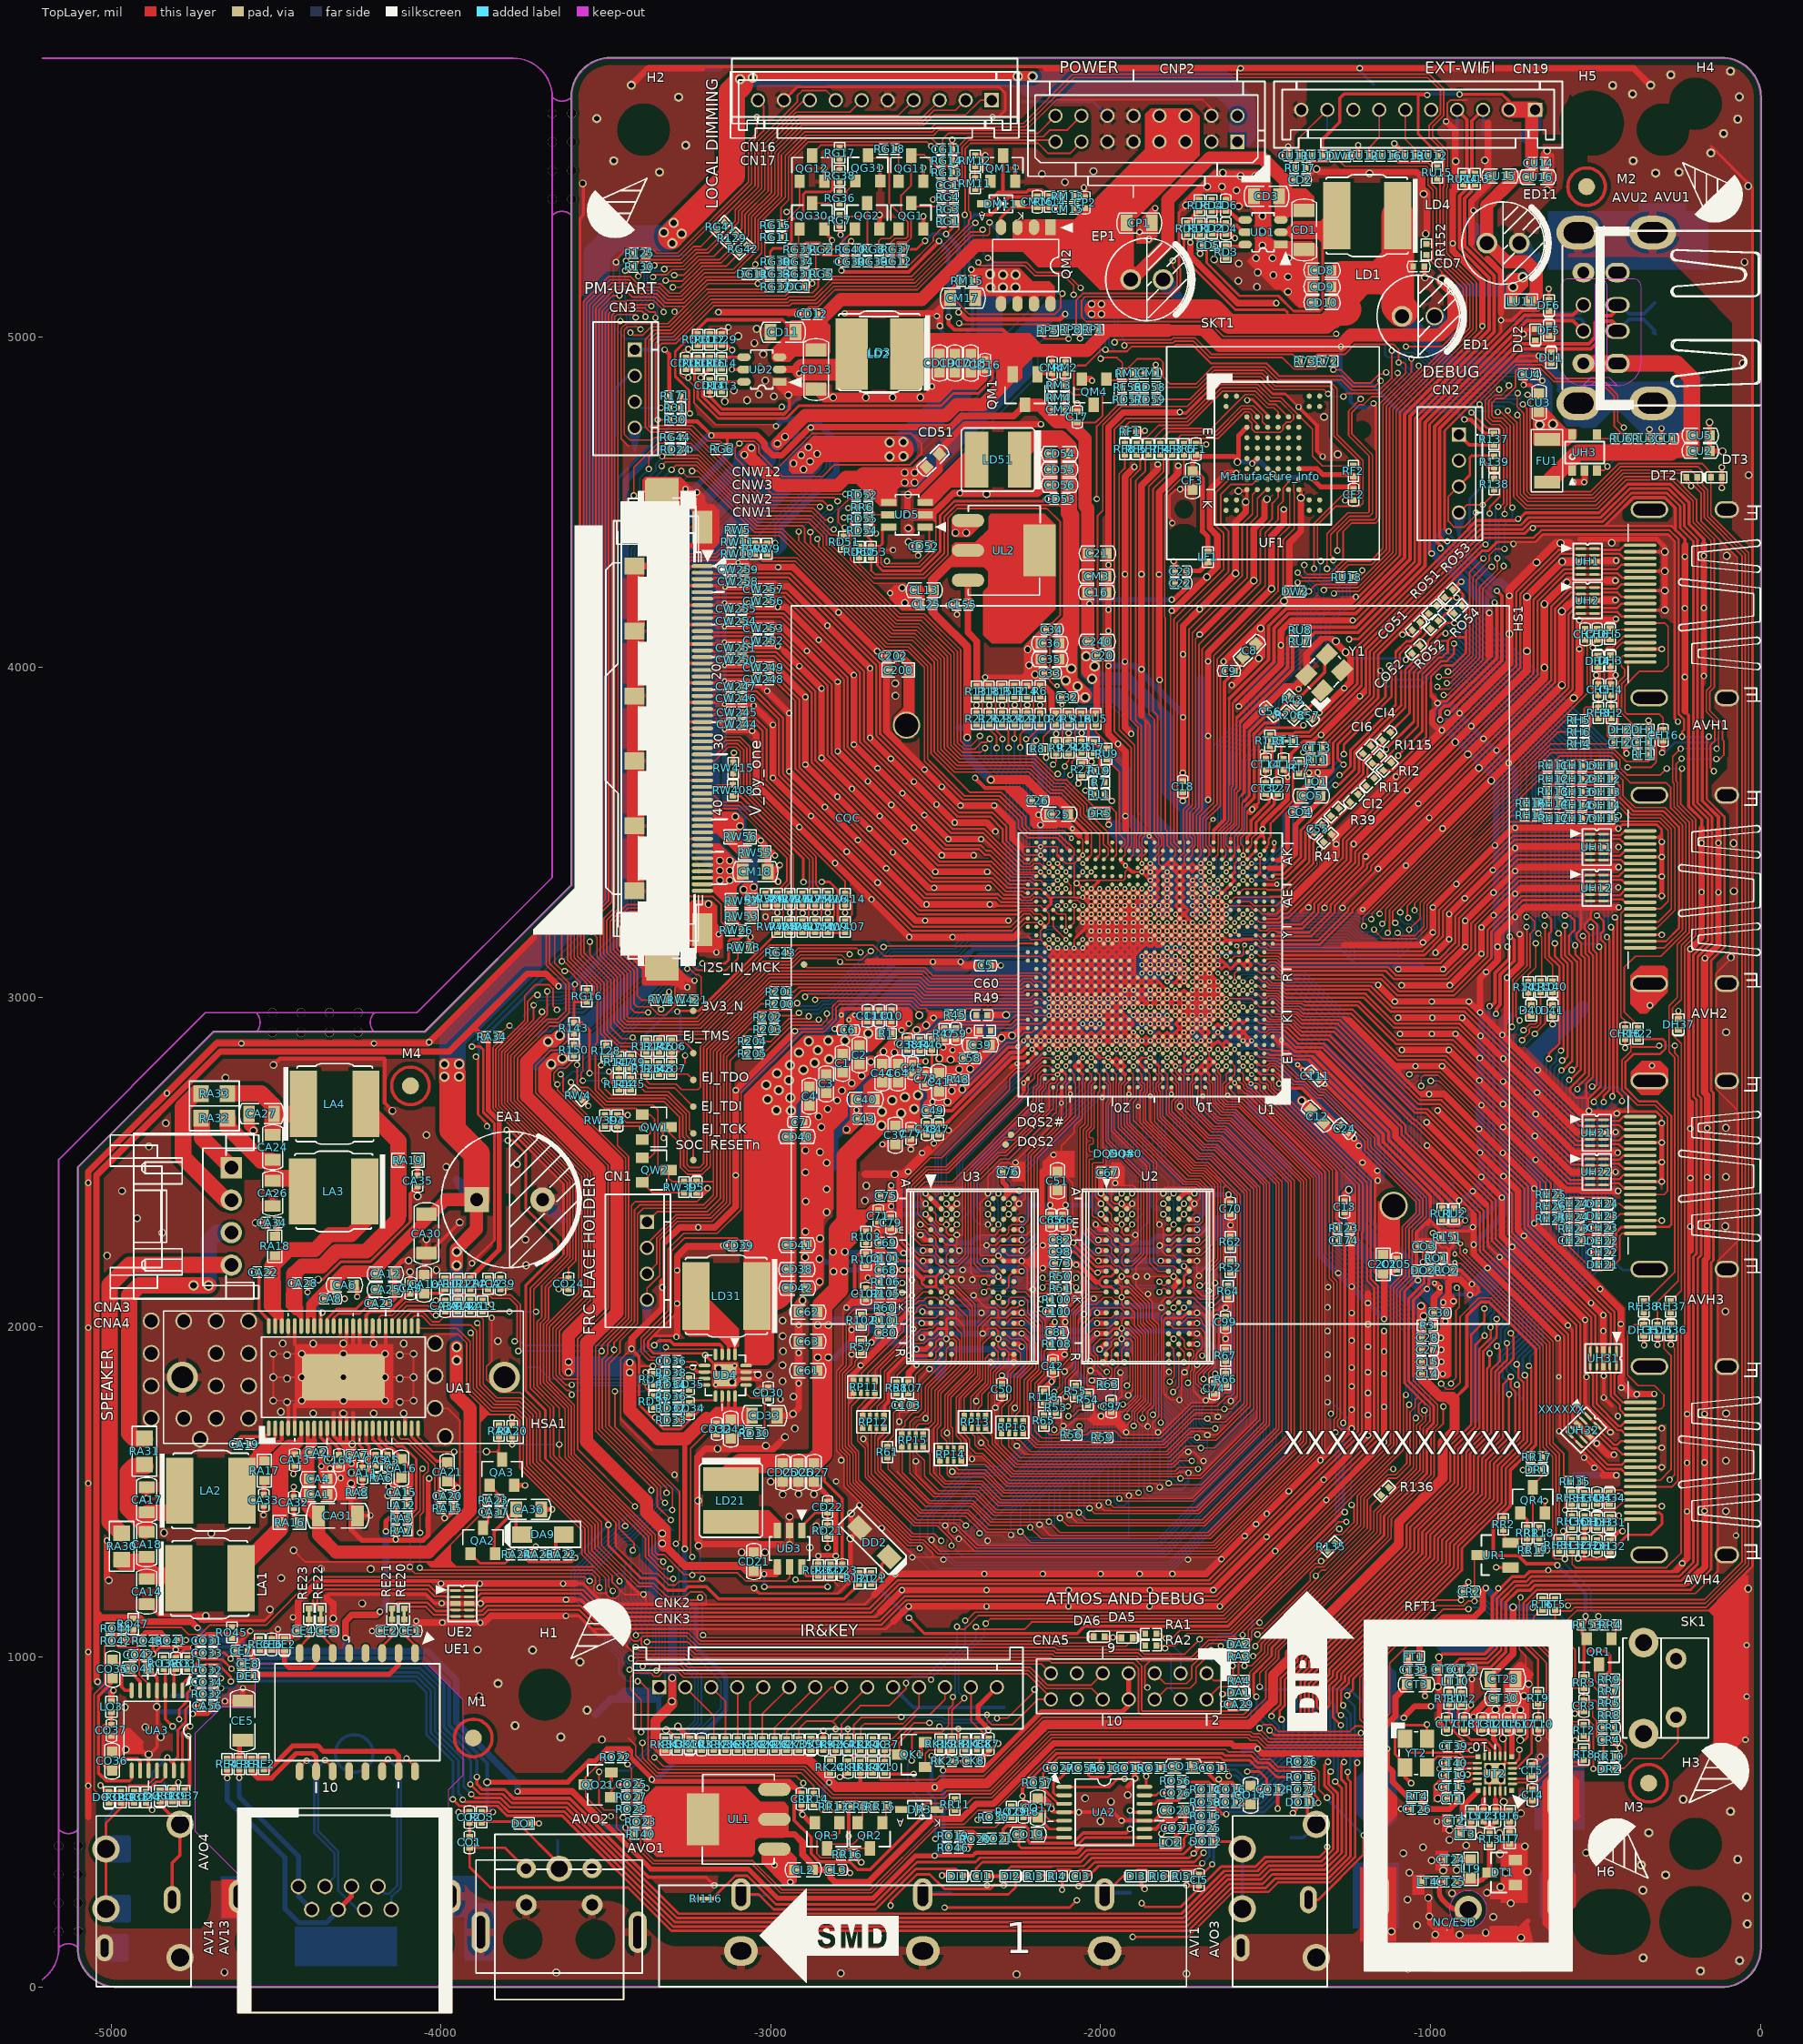
[diagram p0: TopLayer view]
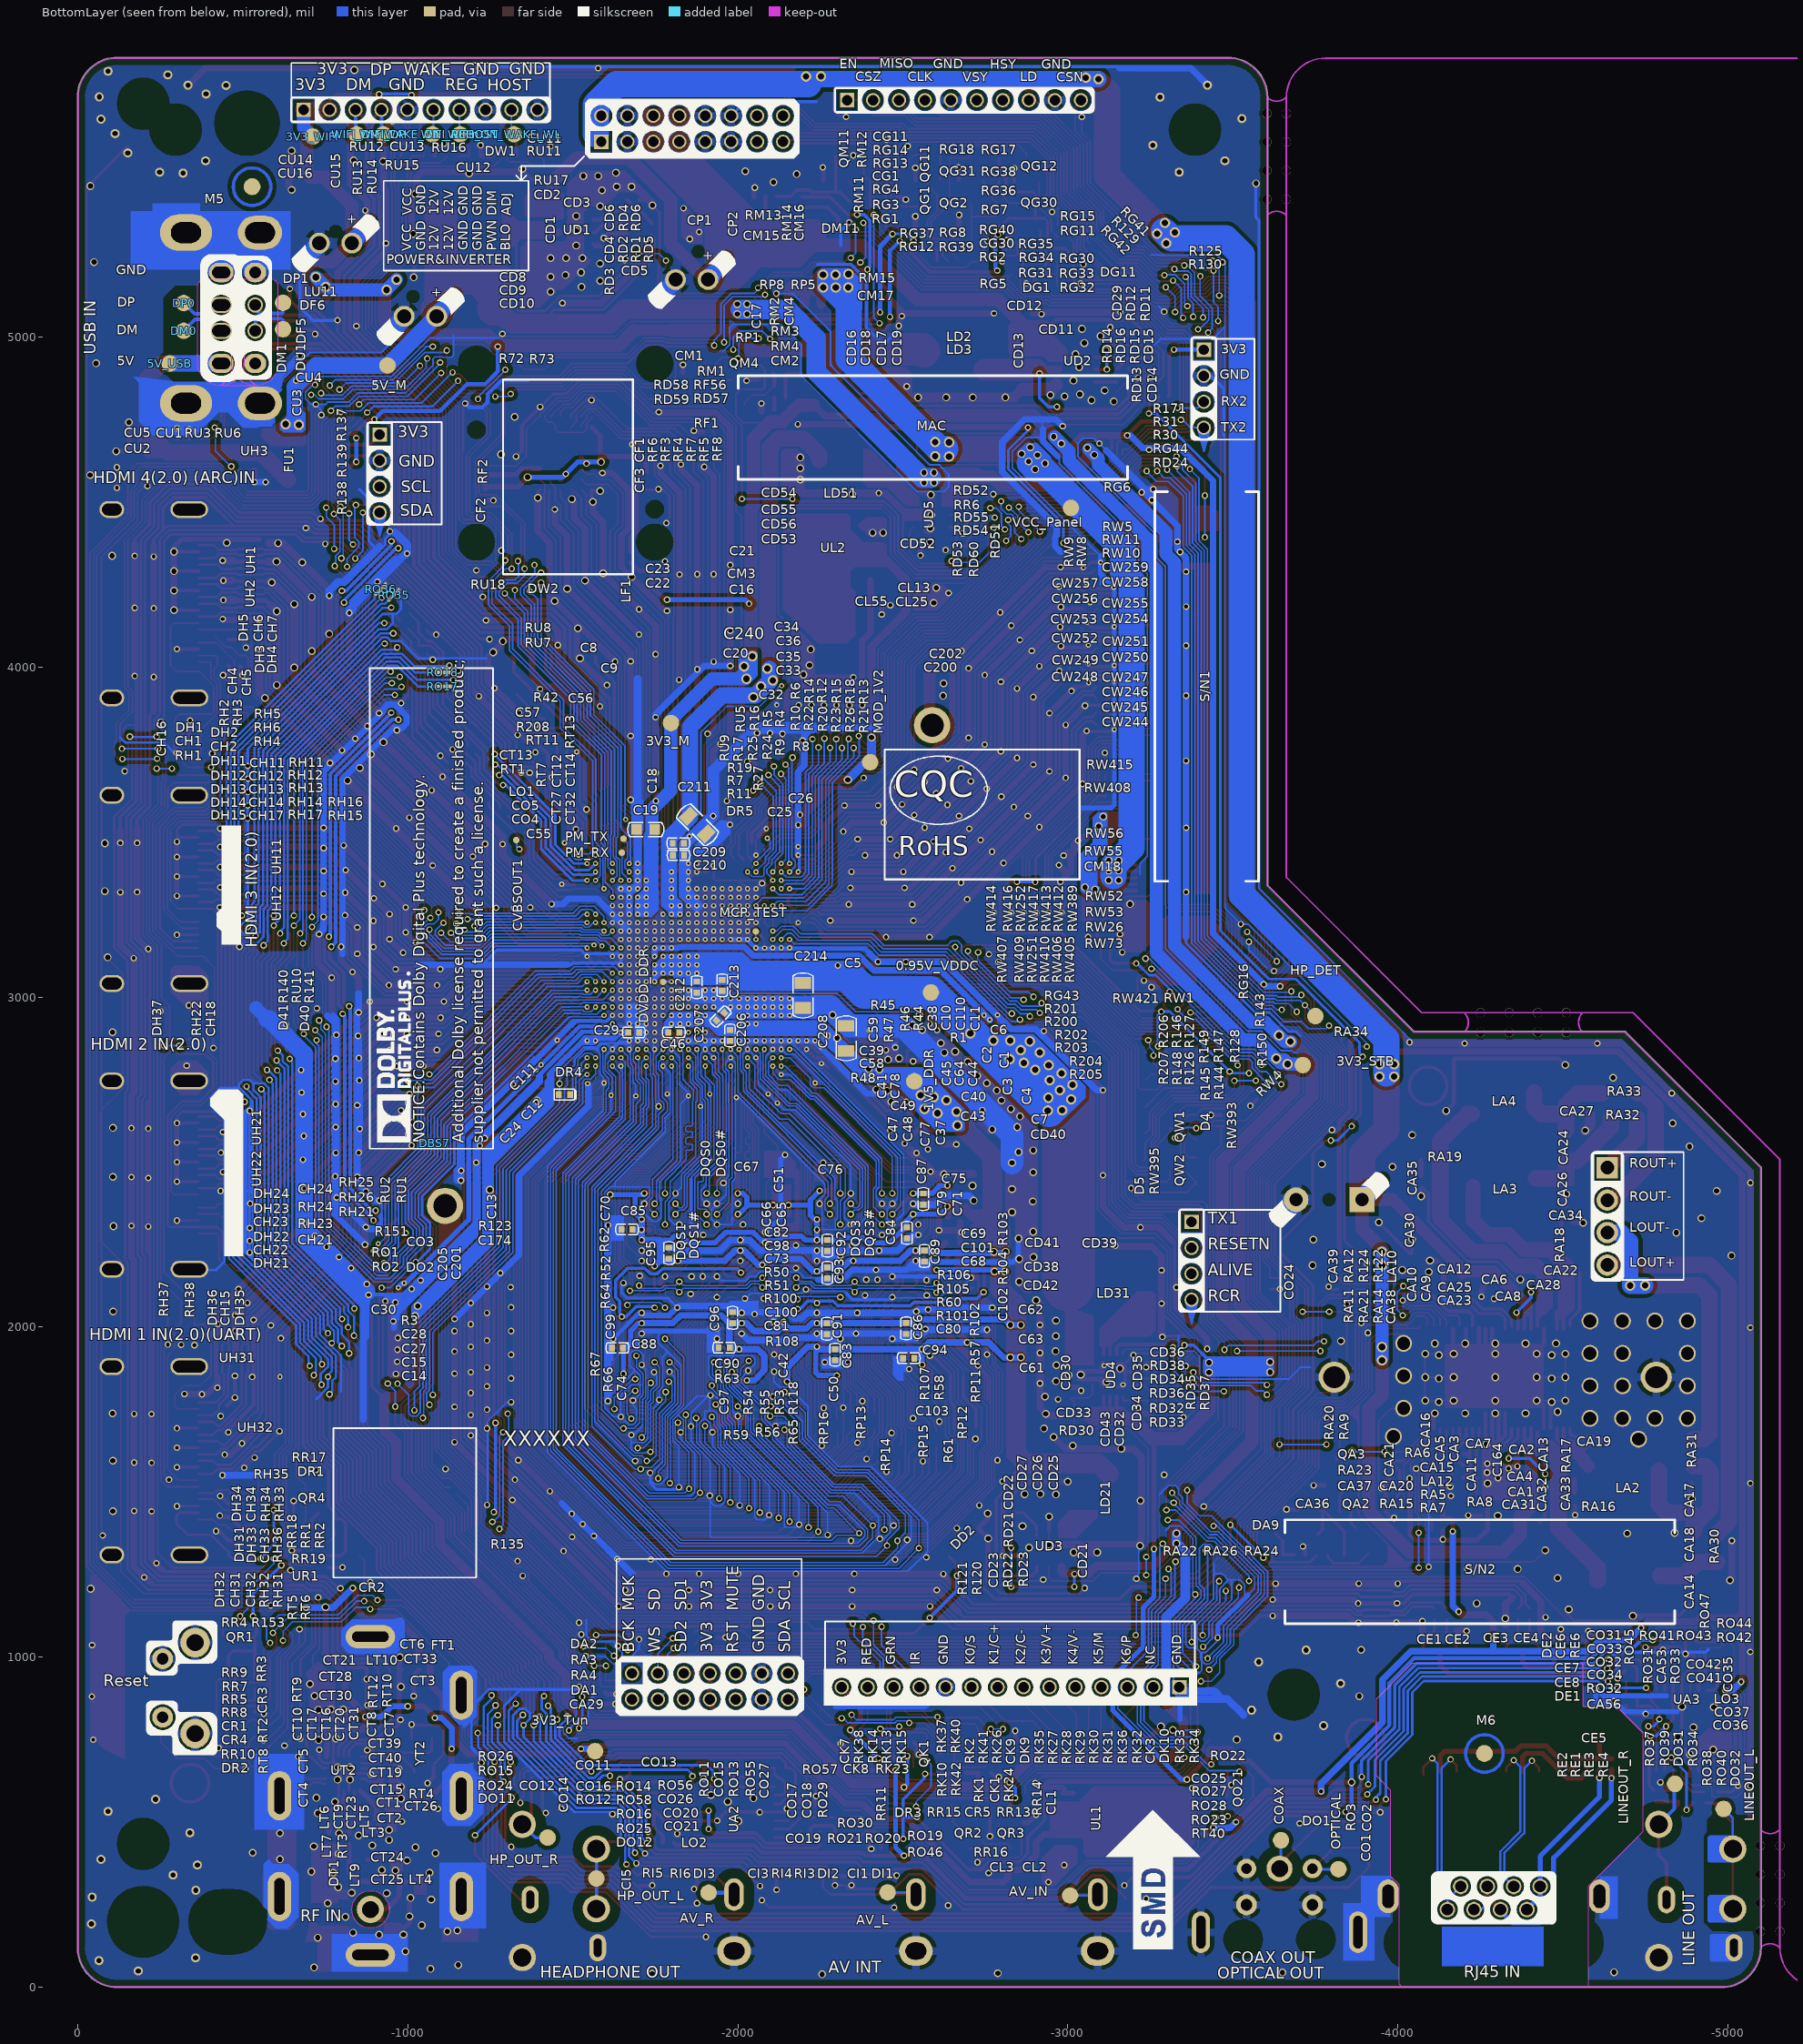
[diagram p1: BottomLayer view, seen from below]
# Altium PCB MISC86290.PcbDoc (part 1 of 31)
Units mil, origin at the board's own origin, x right, y up, seen from the top; angles counter-clockwise.
Board outline 5104.71 x 5851.49 mil, 2 copper layers (TopLayer, BottomLayer), stack 61.855 mil thick; 1026 components, 667 nets, 4280 pads, 2294 vias.

## Layer stack, top to bottom
TopLayer: signal copper 1.4
Dielectric: core 59.055, FR-4, Dk 4.8
BottomLayer: signal copper 1.4

## Board outline
-5102.19,118.11 ccw(c-4981.57,118.11) -4981.57,-2.52 ccw(c-4981.57,0) -4980.94,-2.44 ccw(c-4980.32,0) -4980.32,-2.51 -118.11,-2.51 ccw(c-118.11,0) -118.07,-2.51 ccw(c-118.11,118.11) 2.51,118.07 ccw(c-118.11,118.11) 2.51,118.11 2.51,5728.35 ccw(c-118.11,5728.35) -118.11,5848.97 ccw(c-118.11,5846.46) -118.2,5848.97 -3484.25,5848.97 ccw(c-3484.25,5846.46) -3484.88,5848.89 ccw(c-3485.5,5846.46) -3485.5,5848.97 ccw(c-3485.5,5728.35) -3606.13,5728.35 -3606.13,3339.68 -4049.59,2896.21 -4689.25,2896.21 ccw(c-4689.25,2893.7) -4689.29,2896.21 ccw(c-4689.33,2893.7) -4691.11,2895.48 -5101.45,2485.13 ccw(c-5099.67,2483.36) -5102.19,2483.36 -5102.19,118.23 ccw(c-5099.68,118.11)

## Design rules (kind name [scope] priority, off if disabled: settings)
Clearance ■KEEPOUT_18mil [(IsTrack Or IsArc) And (AsMM(Width) < 1) And IsKeepOut vs Not IsPad] p1: gap=18
Clearance ■DFM_NPTH_10mil [(IsPadHoleValid And (PadIsPlated=false) Or IsPad And ((AsMM(PadXSize_AllLayers) < 1) or (AsMM(PadYSize_AllLayers) < 1 )) And IsKeepout) OR HasFootprintPad('ASSE*','0') vs Not IsPad] p2: gap=10
Clearance ■DFM_20mil [(IsTrack or IsArc or IsPad) And IsKeepOut vs IsTrack or IsArc or InPoly] p3: gap=20
Clearance ■PWR_A12_8mil [(InNetClass('PWR_A12_8mil') or InNet('*12V*') or InNet('*24V*') or InNet('*PVCC*') or InNet('*19V*') or InNet('*AMP*POWER*') or InNet('*AMP*VCC*') or InNet('*LNB*')) and Not IsPad vs Not InPoly] p4: gap=8
Clearance ■SIP2GND_8mil [HasFootprint('SIP*') vs InPoly] p5: gap=8
Clearance ■Poly_4mil [InPolygonClass('Poly_4mil') vs Not InPoly] p6: gap=4
Clearance ■Poly_5mil [InPolygonClass('Poly_5mil') vs Not InPoly] p7: gap=5
Clearance ■Poly_8mil [InPolygonClass('Poly_8mil') vs Not InPoly] p8: gap=8
Clearance ■ESD_10mil [HasFootprint('*IEC*') Or HasFootprint('*-F1*') Or HasFootprint('ANT-RF*')] p9: gap=10
Clearance ■ESD_20mil [HasFootprint('*SHIELD*')] p10: gap=20
Clearance ■C_RFGND_1.8mm [InNet('RFGND') vs Not (InNet('RF*IN*') OR InNet('NetCT28*'))] p11: gap=70.87
Clearance ■GND_12mil [InNet('GND') vs InPoly] p12: gap=12
Clearance ■ESD_30mil [(HasFootprint('SCART*') OR HasFootprint('AV*') OR HasFootprint('DB15*') OR HasFootprint('PHONE*')) vs OnBottomLayer] p13: gap=30
Clearance ■ESD_NT_30mil [HasFootprint('SCART*') Or HasFootprint('PHONE-HD-12') Or HasFootprint('PHONE-HD-17') Or HasFootprint('PHONE-HD-10') Or HasFootprint('PHONE-HD-26') vs InNet('GND') And OnTopLayer] p14: gap=30
Clearance ■DFM_TH_5mil [HasFootprint('GND') or HasFootprint('TP*') or HasFootprint('MARK*') or HasFootprint('SPARK_GAP') or HasFootprint('USB-HD-3-2') or HasFootprint('PHONE-HS-20') and Not IsRegion vs OnBottomlayer And IsPad OR IsPadHoleValid] p15: gap=5
Clearance ■DFM_HS60_5mil [InPadClass('HS60') vs InPadClass('HS60') OR IsPadHoleValid and not InPadClass('VIA5')] p16: gap=5
Clearance ■DFM_BCR_4mm [IsPadHoleValid vs IsBoardCutoutRegion] p17: gap=157.48
Clearance ■DFM_TH_4mm [OnBottomlayer And IsSMTPin vs IsPadHoleValid and not InPadClass('VIA5')] p18: gap=157.48
Clearance ■DFM_HS60_4mm [InPadClass('HS60') vs IsPad and OnBottomlayer] p19: gap=157.48
Clearance ■VIA2VIA_6.2mil [(IsVia OR InPadClass('VIA5')) And Not (IsVia And (AsMM(HoleDiameter) = 0.1)) vs (IsVia OR InPadClass('VIA5')) And Not (IsVia And (AsMM(HoleDiameter) = 0.1))] p20: gap=6.2
Clearance ■VIA2VIA_9.8mil [(IsVia OR InPadClass('VIA5')) And Not (IsVia And (AsMM(HoleDiameter) = 0.1)) vs (IsVia OR InPadClass('VIA5')) And Not (IsVia And (AsMM(HoleDiameter) = 0.1))] p21: gap=9.8
Clearance ■VIA2PAD_BGA_3.9mil [HasFootprint('BGA*') and IsPad vs (IsVia OR InPadClass('VIA5')) And Not (IsVia And (AsMM(HoleDiameter) = 0.1))] p22: gap=3.9
Clearance ■VIA2PAD_5mil [IsVia And Not (IsVia And (AsMM(HoleDiameter) = 0.1)) vs ISPAD and Not HasFootprintPad('*','EPAD') and Not HasFootprintPad('*','257') and Not HasFootprintPad('TP','*') and Not HasFootprintPad('GND','JP*') and Not HasFootprintPad('LQFP216/0.4-2','217') and Not HasFootprintPad('QFP16*','17') and Not HasFootprintPad('QFN16*','17') and Not HasFootprintPad('QFN20*','21') and Not HasFootprintPad('QFN24*','25') and Not HasFootprintPad( 'QFN24*','29') and Not HasFootprintPad('QFN28*','29') and Not HasFootprintPad('QFN32*','33') and Not HasFootprintPad('QFN36*','37') and Not HasFootprintPad('QFN36*','0') and Not HasFootprintPad('QFN32*','0') and Not HasFootprintPad('QFN40*','41') and Not HasFootprintPad('QFN48*','49') and Not HasFootprintPad('LQFP48/0.5-2','49') and Not HasFootprintPad('*SSOP32*','33') and Not HasFootprintPad('SOP8*','9') and Not HasFootprintPad('WSON8/1.27*','9') and Not HasFootprintPad('DFN10/0.5-1*','11') and Not HasFootprintPad('SON16/0.4','9') and Not HasFootprintPad('MSOP10/0.5-1','11') and Not HasFootprintPad('QFN56/0.5','57') and Not HasFootprintPad('LGA31/0.5','3*') and Not InPadClass('VIA_HS60') and Not HasFootprintPad('TSSOP16/0.65-3','17') and Not HasFootprintPad('QFP128/0.5-2','129') and Not HasFootprintPad('QFP128/0.4-5','129') and Not HasFootprintPad('PQFP48*','49') and Not HasFootprintPad('QFP156/0.4-1','157')] p23: gap=5
Clearance ■PAD2VIA5_6mil [IsPad And ((AsMM(PadXSize_AllLayers) < 2.5) or ((AsMM(PadYSize_AllLayers) < 2.5))) And Not InPadclass('HS60') vs InPadClass('VIA5')] p24: gap=6
Clearance "■12mil for Polygon" [InPoly] p25: gap=12
Clearance 8mil [All] p26 off: gap=8
Clearance 7mil [All] p27 off: gap=7
Clearance 6.2mil [All] p28 off: gap=6.2
Clearance 6mil [All] p29 off: gap=6
Clearance 5.8mil [All] p30 off: gap=5.8
Clearance 5mil [Not ((IsTrack Or IsArc) And (Layer = 'KeepOutLayer')) vs Not (IsPad or ((IsTrack Or IsArc) And (Layer = 'KeepOutLayer')))] p31 off: gap=5
Clearance 4.5mil [Not ((IsTrack Or IsArc) And (Layer = 'KeepOutLayer')) vs Not (IsPad or ((IsTrack Or IsArc) And (Layer = 'KeepOutLayer')))] p32 off: gap=4.5
Clearance "3.9mil for Minimum" [Not ((IsTrack Or IsArc) And (Layer = 'KeepOutLayer')) vs Not (IsPad or ((IsTrack Or IsArc) And (Layer = 'KeepOutLayer')))] p33: gap=3.9
ComponentClearance [All] p1 off: gap=0.1 collisioncheckmode=3 verticalgap=39.37 showdistances=FALSE
DiffPairsRouting DiffPair_USB_DiffPairsRouting [InDifferentialPairClass('USB')] p1: maxlimit=5 minlimit=4 mostfreqgap=5 maxuncoupledlength=200
DiffPairsRouting DiffPair_LVDS_DiffPairsRouting [InDifferentialPairClass('LVDS')] p2: maxlimit=5 minlimit=4 mostfreqgap=5 maxuncoupledlength=500
DiffPairsRouting DiffPair_HDMI_DiffPairsRouting [InDifferentialPairClass('HDMI')] p3: maxlimit=5 minlimit=4 mostfreqgap=5 maxuncoupledlength=200
DiffPairsRouting [All] p4: maxlimit=10 minlimit=10 mostfreqgap=10 maxuncoupledlength=500
FabricationTestPointUsage TestPointUsage [All] p1: valid=0 allowmultiple=FALSE
FabricationTestpoint Testpoint [All] p1: side=3 testpointundercomponent=TRUE minsize=40 maxsize=100 preferedsize=60 minholesize=20 maxholesize=40 preferedholesize=32 testpointgrid=1 allowsidetop=TRUE allowsidebottom=TRUE usegrid=TRUE gridtolerance=0.01
HoleSize HoleSize_VIA [ISVIA] p1 off: absolutevalues=TRUE maxlimit=23.62 minlimit=7.87 maxpercent=80.000 minpercent=20.000
HoleToHoleClearance Hole2Hole [All] p1 off: gap=18 allowstackedmicrovias=FALSE
MatchedLengths DiffPair_USB_MatchedLengths [InDifferentialPairClass('USB')] p1: tolerance=100 checknetsindiffpair=TRUE checkdiffpairvsdiffpair=FALSE checkothers=FALSE
MatchedLengths DiffPair_LVDS_MatchedLengths [InDifferentialPairClass('LVDS')] p2: tolerance=100 checknetsindiffpair=TRUE checkdiffpairvsdiffpair=FALSE checkothers=FALSE
MatchedLengths DiffPair_HDMI_MatchedLengths [InDifferentialPairClass('HDMI')] p3: tolerance=100 checknetsindiffpair=TRUE checkdiffpairvsdiffpair=FALSE checkothers=FALSE
MinimumAnnularRing [All] p1: minimumring=3.94
MinimumSolderMaskSliver [All] p1 off: minsoldermaskwidth=-1
NetAntennae [Not (HasFootprint('ANT-7') or HasFootprint('ANT-BLUECORE'))] p1: netantennaetolerance=40
PermittedLayers [All] p1: toplayerpermitted=TRUE bottomlayerpermitted=TRUE
PlaneClearance Plane_ESD_30mil [(HasFootprint('SCART*') OR HasFootprint('AV*') OR HasFootprint('DB15*') OR HasFootprint('PHONE*'))] p1: clearance=30
PlaneClearance [All] p2: clearance=9
PlaneConnect Plane2Via [IsVia or InPadClass('VIA5')] p1: planeconnectstyle=Direct reliefexpansion=20 reliefentries=4 reliefconductorwidth=10 reliefairgap=10
PlaneConnect PlaneConnect_PAD [HasFootprint('ASSE*') OR InPadclass('HS60')] p2: planeconnectstyle=Direct reliefexpansion=20 reliefentries=4 reliefconductorwidth=10 reliefairgap=10
PlaneConnect [All] p3: planeconnectstyle=Relief reliefexpansion=12 reliefentries=4 reliefconductorwidth=30 reliefairgap=12
PolygonConnect PourOverVia [IsVia vs IsPolygon] p1: connectstyle=Direct reliefconductorwidth=10 reliefentries=4 polygonreliefangle="90 Angle"
PolygonConnect VIA5_HS60 [InPadclass('HS60') or InPadClass('VIA5') vs IsPolygon] p2: connectstyle=Direct reliefconductorwidth=10 reliefentries=4 polygonreliefangle="90 Angle"
PolygonConnect Polygon_RFGND [InNet('RFGND')] p3: connectstyle=Direct reliefconductorwidth=10 reliefentries=4 polygonreliefangle="90 Angle"
PolygonConnect ESD_SCART [HasFootprint('SCART*') vs IsPolygon And onBottomlayer] p4: connectstyle=Direct reliefconductorwidth=30 reliefentries=4 polygonreliefangle="90 Angle"
PolygonConnect FH2Polygon [HasFootprint('ASSE*') or HasFootprint('DIODE-S0402') or HasFootprint('RCL0524P') vs IsPolygon] p5: connectstyle=Direct reliefconductorwidth=10 reliefentries=4 polygonreliefangle="90 Angle"
PolygonConnect PWC1_2Polygon [(HasFootprint('*0805*') OR HasFootprint('*1206*')) vs IsPolygon] p6: connectstyle=Relief reliefconductorwidth=30 reliefentries=4 polygonreliefangle="90 Angle"
PolygonConnect PWC2_2Polygon [HasFootprint('*0603*') vs IsPolygon] p7: connectstyle=Relief reliefconductorwidth=25 reliefentries=4 polygonreliefangle="90 Angle"
PolygonConnect PWC3_2Polygon [HasFootprint('EC*') vs IsPolygon] p8: connectstyle=Relief reliefconductorwidth=35 reliefentries=4 polygonreliefangle="90 Angle"
PolygonConnect PWC2Polygon [(HasFootprint('SOT-89') OR HasFootprint('SOT-223') OR HasFootprint('TO-252') OR HasFootprint('TO-263') OR HasFootprint('DIODE') OR HasFootprint('SW-HS-2') OR HasFootprint('HDMI*') OR HasFootprint('SO-8B') OR HasFootprint('GND') OR HasFootprint('PHONE*') OR HasFootprint('DIP18/2.54-2') OR HasFootprint('DIP18/2.54-1') OR HasFootprint('UFL-R-SMT-1') OR HasFootprint('WIFI') OR HasFootprint('UM02BS') OR HasFootprint('*SCART*') OR HasFootprint('TSOT23-8/0.65') OR HasFootprint('*SOT-23-*') OR HasFootprint('SOP23-5-1') OR HasFootprint('SOP6/0.95') OR HasFootprint('M-WIFI-2-M603USA1') OR HasFootprint('M-MT7632U') OR HasFootprint('SOP8/1.27') OR HasFootprint('SOP8/1.27-3')) vs IsPolygon] p9: connectstyle=Direct reliefconductorwidth=35 reliefentries=4 polygonreliefangle="90 Angle"
PolygonConnect SMD2Polygon [IsSMTPin vs IsPolygon] p10: connectstyle=Relief reliefconductorwidth=12 reliefentries=4 polygonreliefangle="90 Angle"
PolygonConnect PTH2Polygon [IsThruPin vs IsPolygon] p11: connectstyle=Relief reliefconductorwidth=25 reliefentries=4 polygonreliefangle="90 Angle"
RoutingVias 0.6_0.4 [All] p1 off: holewidth=15.75 width=23.62 viastyle="Through Hole" minholewidth=15.75 minwidth=23.62 maxholewidth=15.75 maxwidth=23.62
RoutingVias 0.8_0.5 [All] p2 off: holewidth=19.68 width=31.5 viastyle="Through Hole" minholewidth=19.68 minwidth=31.5 maxholewidth=19.68 maxwidth=31.5
RoutingVias 0.5_0.3 [All] p3: holewidth=11.81 width=19.68 viastyle="Through Hole" minholewidth=11.81 minwidth=19.68 maxholewidth=11.81 maxwidth=19.68
RoutingVias 0.45_0.25 [All] p4 off: holewidth=9.84 width=17.72 viastyle="Through Hole" minholewidth=9.84 minwidth=17.72 maxholewidth=9.84 maxwidth=17.72
RoutingVias 0.4_0.2 [All] p5: holewidth=7.87 width=15.75 viastyle="Through Hole" minholewidth=7.87 minwidth=15.75 maxholewidth=7.87 maxwidth=15.75
RoutingVias 0.25_0.1 [All] p6 off: holewidth=3.94 width=9.84 viastyle="Through Hole" minholewidth=3.94 minwidth=9.84 maxholewidth=3.94 maxwidth=9.84
SMDNeckDown SMDNeckDown_Chip [HasFootprint('FFC*') or HasFootprint('QFP*') or HasFootprint('QFN*') or HasFootprint('HDMI*') or HasFootprint('BGA*')] p1: percent=100.000
SMDToCorner [All] p1 off: distance=40000
ShortCircuit ■ShortCircuit_ViaOnEpad [HasFootprintPad( '*','EPAD') vs IsVia AND InNet('*')] p1: allowed=TRUE
ShortCircuit ■ShortCircuit_JP [HasFootprintPad( 'GND','JP_1K') vs HasFootprintPad( 'GND','JP_2K')] p2: allowed=TRUE
ShortCircuit ■ShortCircuit_0402 [HasFootprintPad('R0402SC','1') OR HasFootprintPad('R0402SC','2') vs HasFootprintPad('R0402SC','3')] p3: allowed=TRUE
ShortCircuit ■ShortCircuit [InNet('*')] p4: allowed=FALSE
SilkToSilkClearance Silk2Silk [All] p1: silktosilkclearance=5
SilkscreenOverComponentPads [IsText] p1: minsilkscreentomaskgap=0.1
SolderMaskExpansion SolderMask_BGA [HasFootprint('BGA*') OR HasFootprint('*0201*')] p1: expansion=2
SolderMaskExpansion SolderMask_VIA [IsVia] p2: expansion=5.1
SolderMaskExpansion [All] p3: expansion=3
UnRoutedNet ■UnRoutedNet [All] p1:
ViasUnderSMD [All] p1: allowed=FALSE
Width DiffPair_USB_Width [InDifferentialPairClass('USB')] p1: maxlimit=11 minlimit=4 preferedwidth=11
Width DiffPair_LVDS_Width [InDifferentialPairClass('LVDS')] p2: maxlimit=7 minlimit=4 preferedwidth=7
Width DiffPair_HDMI_Width [InDifferentialPairClass('HDMI')] p3: maxlimit=7 minlimit=4 preferedwidth=7
Width [All] p4: maxlimit=250 minlimit=3 preferedwidth=8
14 further rules are at their usual default settings.

## Classes and differential pairs
component class TV#14_WIFI&LOCAL_DIMMING: 3V3_WIFI CN16 CN17 CN19 CU11 CU12 CU13 CU14 CU15 CU16 DW1 DW2 ED11 HOST_WAKE_WL LU11 RG41 RG42 RU11 RU12 RU13 RU14 RU15 RU16 RU17 WAKE_ON_WIFIn WIFI_DM WIFI_DP WIFI_REG_ON
component class TV#13_TUNER_SI2151: CT1 CT2 CT3 CT4 CT5 CT6 CT7 CT8 CT9 CT10 CT12 CT13 CT14 CT15 CT16 CT17 CT19 CT20 CT21 CT23 CT24 CT25 CT26 CT27 CT28 CT30 CT31 CT32 CT33 CT39 CT40 DT1 DT2 DT3 FT1 LT3 LT4 LT5 LT6 LT7 LT9 LT10 NC/ESD RFT1 RT1 RT2 RT3 RT4 RT5 RT6 RT7 RT8 RT9 RT10 RT11 RT12 RT13 RT40 UT2 YT2
component class TV#12_AMP_TAS5751M: C164 CA1 CA2 CA3 CA4 CA5 CA6 CA7 CA8 CA9 CA10 CA11 CA12 CA13 CA14 CA15 CA16 CA17 CA18 CA19 CA20 CA21 CA22 CA23 CA24 CA25 CA26 CA27 CA28 CA29 CA30 CA31 CA32 CA33 CA34 CA35 CA38 CA39 CNA3 CNA4 CNA5 DA1 DA2 DA5 DA6 EA1 HSA1 LA1 LA2 LA3 LA4 LA10 LA12 RA1 RA2 RA3 RA4 RA5 RA6 RA7 RA8 RA9 RA11 RA12 RA14 RA15 RA16 RA17 RA18 RA19 RA20 RA21 RA30 RA31 RA32 RA33 RA34 UA1
component class TV#11_USB&RJ45: 5V_USB AV13 AV14 AVU1 AVU2 CE1 CE2 CE3 CE4 CE5 CE6 CE7 CE8 CU1 CU2 CU3 CU4 CU5 DE1 DE2 DF5 DF6 DM0 DM1 DP0 DP1 DU1 DU2 FU1 RE1 RE2 RE3 RE4 RE6 RE20 RE21 RE22 RE23 RU1 RU2 RU3 RU5 RU6 RU7 RU8 UE1 UE2 UH3
component class TV#10_HDMI: AVH1 AVH2 AVH3 AVH4 CH1 CH2 CH4 CH5 CH6 CH7 CH11 CH12 CH13 CH14 CH15 CH17 CH18 CH21 CH22 CH23 CH24 CH31 CH32 CH33 CH34 DH1 DH2 DH3 DH4 DH5 DH11 DH12 DH13 DH14 DH15 DH21 DH22 DH23 DH24 DH31 DH32 DH33 DH34 DH35 DH36 RH1 RH2 RH3 RH4 RH5 RH6 RH11 RH12 RH13 RH14 RH15 RH16 RH17 RH21 RH22 RH23 RH24 RH25 RH26 RH31 RH32 RH33 RH34 RH35 RH36 RH37 RH38 UH1 UH2 UH11 UH12 UH21 UH22 UH31 UH32
component class TV#09_AV&SPDIF&LINEOUT&HEADPHONE: AV_IN AV_L AV_R AVI1 AVO1 AVO2 AVO3 AVO4 CA53 CA56 CI1 CI2 CI3 CI4 CI5 CI6 CO1 CO2 CO3 CO11 CO12 CO13 CO14 CO16 CO17 CO18 CO19 CO20 CO21 CO24 CO25 CO27 CO31 CO32 CO33 CO34 CO35 CO36 CO37 CO41 CO42 COAX DI1 DI2 DI3 DO1 DO2 DO11 DO12 DO31 DO32 HP_DET HP_OUT_L HP_OUT_R LINEOUT_L LINEOUT_R LO2 LO3 OPTICAL QO21 RI1 RI2 RI3 RI4 RI5 RI6 RO1 RO2 RO3 RO11 RO12 RO13 RO14 RO15 RO16 RO17 RO18 RO19 RO20 RO21 RO22 RO23 RO24 RO25 RO26 RO27 RO28 RO29 RO30 RO31 RO32 RO33 RO34 RO35 RO36 RO37 RO38 RO39 RO40 RO41 RO42 RO43 RO44 RO45 UA2 UA3
component class TV#08_KEY&LED&IR: CK1 CK3 CK7 CK8 CK9 CNK2 CNK3 DK9 DK10 QK1 RK1 RK2 RK10 RK13 RK14 RK15 RK23 RK24 RK26 RK27 RK28 RK29 RK30 RK31 RK32 RK33 RK34 RK35 RK36
component class TV#07_VB1: CNW1 CNW2 CNW3 CNW12 CW244 CW245 CW246 CW247 CW248 CW249 CW250 CW251 CW252 CW253 CW254 CW255 CW256 CW257 CW258 CW259 QW1 QW2 RW1 RW4 RW8 RW9 RW10 RW11 RW26 RW52 RW53 RW55 RW56 RW73 RW251 RW252 RW389 RW393 RW395 RW405 RW406 RW407 RW408 RW409 RW410 RW412 RW413 RW414 RW415 RW416 RW417 RW421
component class TV#06_DDR: C58 C59 C60 C61 C62 C63 C64 C65 C66 C67 C68 C69 C70 C71 C73 C74 C75 C76 C77 C78 C79 C80 C81 C82 C83 C84 C85 C86 C87 C88 C89 C90 C91 C92 C93 C94 C95 C96 C97 C98 C99 C100 C101 C102 C103 DQS0 DQS0# DQS1 DQS1# DQS2 DQS2# DQS3 DQS3# MCP_TEST R44 R45 R46 R47 R48 R49 R50 R51 R52 R53 R54 R55 R56 R57 R58 R59 R60 R61 R62 R63 R64 R65 R66 R67 R100 R101 R102 R103 R104 R105 R106 R107 R108 R118 RP11 RP12 RP13 RP14 RP15 RP16 U1 U2 U3
component class TV#05_NAND_FLASH: CF1 CF2 CF3 LF1 R4 R5 R6 R7 R8 R9 R10 R11 R12 R13 R14 R15 R16 R17 R18 R19 R20 R21 R22 R23 R24 R25 R26 R27 RF1 RF2 RF3 RF4 RF5 RF6 RF7 RF8 SKT1 UF1
component class TV#04_SOC_SYSTEM: C55 C56 C57 C174 CN1 CN2 CO4 CO5 CO51 CO52 CR1 CR2 CR3 CR4 CR5 CVBSOUT1 D4 D5 D40 D41 DD2 DR1 DR2 DR3 DR4 DR5 EJ_TCK EJ_TDI EJ_TDO EJ_TMS I2S_IN_MCK LO1 QR1 QR2 QR3 QR4 R30 R31 R39 R41 R42 R72 R73 R120 R121 R122 R123 R124 R125 R126 R127 R128 R129 R130 R135 R136 R137 R138 R139 R140 R141 R143 R144 R145 R146 R147 R148 R149 R150 R151 R152 R153 RI115 RI116 RO51 RO52 RO53 RO54 RR1 RR2 RR3 RR4 RR5 RR6 RR7 RR8 RR9 RR10 RR11 RR13 RR14 RR15 RR16 RR17 RR18 RR19 SK1 SOC_RESETn UR1 Y1
component class TV#02_SOC_POWER: C1 C2 C3 C4 C5 C6 C7 C8 C9 C10 C11 C12 C13 C15 C16 C17 C18 C19 C20 C21 C22 C23 C24 C25 C26 C27 C28 C29 C30 C31 C32 C33 C34 C35 C36 C37 C38 C39 C40 C41 C42 C43 C44 C45 C46 C47 C48 C49 C50 C51 C110 C111 C206 C207 C208 C209 C210 C211 C212 C213 C214 DVDD_DDR R1 R2 R3
component class TV#01_SYSTEM_POWER: 0.95V_VDDC 1V5_DDR 3V3_M 3V3_STB 3V3_Tun 5V_M CD1 CD2 CD3 CD4 CD5 CD6 CD7 CD8 CD9 CD10 CD11 CD12 CD13 CD14 CD15 CD16 CD17 CD18 CD19 CD21 CD22 CD23 CD25 CD26 CD27 CD29 CD30 CD32 CD33 CD34 CD35 CD36 CD38 CD39 CD40 CD41 CD42 CD43 CD51 CD52 CD53 CD54 CD55 CD56 CG1 CG11 CG30 CL1 CL2 CL3 CL13 CL25 CL55 CM1 CM2 CM3 CM4 CM15 CM16 CM17 CM18 CNP2 CP1 CP2 DG1 DG11 DM11 ED1 EP1 LD1 LD2 LD3 LD4 LD21 LD31 LD51 MOD_1V2 QG1 QG2 QG11 QG12 QG30 QG31 QM1 QM2 QM4 QM11 RD1 RD2 RD3 RD4 RD5 RD6 RD11 RD12 RD13 RD14 RD15 RD16 RD21 RD22 RD23 RD24 RD30 RD32 RD33 RD34 RD35 RD36 RD37 RD38 RD51 RD52 RD53 RD54 RD55 RD57 RD58 RD59 RF56 RG1 RG2 RG3 RG4 RG5 RG6 RG7 RG8 RG11 RG12 RG13 RG14 RG15 RG16 RG17 RG18 RG30 RG31 RG32 RG33 RG34 RG35 RG36 RG37 RG38 RG39 RG40 RM1 RM2 RM3 RM4 RM11 RM12 RM13 RM14 RM15 RP1 RP5 RP8 UD1 UD2 UD3 UD4 UD5 UL1 UL2 VCC_Panel
component class "TV#00_Block Diagram": * IR&KEY MAINBOARD
component class SCH_info: C200 C201 C202 C205 HS1 P1(用于U1上) XXXXXX XXXXXXXXXXX
component class PCB_info: A13XX AI_V Barcode CAUTION COLD CQC DIP H1 H2 H3 H4 H5 H6 "High Voltage" HOT M1 M2 M3 M4 M5 M6 MAC Manufacture_Info S/N1 S/N2 SMD
pad class VIA5: C4-1 C16-1 C18-2 C19-1 C20-2 C21-1 C33-2 C34-2 C35-1 C36-1 C37-2 C40-1 C44-1 C61-1 C62-1 C63-1 C64-1 C103-1 CD25-1 CD26-1 CD27-1 CD30-1 CD32-1 CD33-2 CD38-1 CD40-1 CD41-1 CD42-1 CD43-1 CE5-2 CF3-1 CM3-1 CO36-1 CO37-1 DD2-A Free-VIA5 UD4-14 UD4-15
pad class ShortCricuit_JP2: GND_JP1-JP_2K GND_JP2-JP_2K
pad class ShortCricuit_JP1: GND_JP1-JP_1K GND_JP2-JP_1K
polygon class Poly_5mil: 5 5mil

## Components (designator, comment, footprint, x,y, rotation, side; value= is the part's Value field where it differs from the comment)
0.95V_VDDC "TEST" TP -2585,3014 r90 bottom
1V5_DDR "TEST" TP -2534.76,2744.88 r270 bottom
3V3_M "TEST" TP -1797,3831 r180 bottom
3V3_N "TEST" TP-20#1 -3235.5,2958.5 r90 top
3V3_STB "TEST" TP -3712.5,2794 r180 bottom
3V3_Tun "TEST" TP -1567,714 r315 bottom
3V3_WIFI "TEST" TP -711,5609 r90 bottom
5V_M "TEST" TP -937.46,4915 r180 bottom
5V_USB "TEST" TP -277.25,4921 r90 bottom locked
AI_V "AI_GRIPPER_V" AI_GRIPPER_V 1079,-1456 r270 top
AV13 "NC/Network terminal,Network Terminal,DIP,5631-S-F-8C-1E-01,GLGNET" RJ45U-D-5 -4291.39,-78.74 r0 top locked
AV14 "Network terminal,Network Terminal,DIP,WLRJ-277A,WLCO" RJ45U-D-14 -4291.39,0 r0 top locked
AV_IN "TEST" TP -3006.75,276.5 r90 bottom
AV_L "TEST" TP -2453.5,286 r180 bottom
AV_R "TEST" TP -1911,285 r180 bottom
AVH1 "161011041" HDMI-HS-1 78.74,4192.92 r90 top locked
AVH2 "161011041" HDMI-HS-1 78.74,3326.77 r90 top locked
AVH3 "161011041" HDMI-HS-1 78.74,2460.63 r90 top locked
AVH4 "161011041" HDMI-HS-1 78.74,1594.49 r90 top locked
AVI1 "RCA jack,RCA Jack,AV3,H,Yellow,White,Red,CH5.5,D14,Seal,DIP,AV3-8.4-15C,JSL(MI material)" AV3-H14-15 -2539.37,0 r0 top locked
AVO1 "NC/RCA jack,RCA Jack,AV1,H,Orange,CH5.5,Seal,DIP,AV38A-01S-5020,QS" AV1-H-4 -3641.74,41.34 r0 top locked
AVO2 "Optical terminal,OPTICAL,H,DIP,DQT-015B1,DQ" OPTICAL-HD-6 -3641.74,-39.37 r0 top locked
AVO3 "Earphone terminal,Earphone Jack,H,Φ3.5,CH7.0,Black,switch,Seal,DIP,PJ-373A,JSL" PHONE-HD-42 -1456.7,0 r0 top locked
AVO4 "Earphone terminal,Earphone Jack,H,Φ3.5,CH7.0,Black,switch,Seal,DIP,PJ-373A,JSL" PHONE-HD-42 -4901.57,0 r0 top locked
AVU1 "NC/USB terminal,USB Jack,H,Single,flange,DIP,WLUS-050F USB,WLCO" USB1-HD-2 76.68,5059.04 r90 top locked
AVU2 "WLUS-074B" USB2-HD-1 78.76,5059.04 r90 top locked
C1 "Ceramic capacitor,CAP MC,6.3V,22uF,±20%,X5R,0603,SMD,TP" C0603 -2783,2799.81 r90 top
C2 "Ceramic capacitor,CAP MC,6.3V,10uF,±20%,X5R,0603,SMD,TP" C0603 -2731.5,2825.31 r90 top
C3 "Ceramic capacitor,CAP MC,6.3V,10uF,±20%,X5R,0603,SMD,TP" C0603 -2832,2737.31 r90 top
C4 "Ceramic capacitor,CAP MC,6.3V,10uF,±20%,X5R,0603,SMD,TP" C0603 -2883,2699.81 r90 top
C5 "0.1uF-0402-X5R-±20%-16V" C0402#1 -2349,3096 r180 top
C6 "0.1uF-0402-X5R-±20%-16V" C0402#1 -2765.23,2900.5 r180 top
C7 "0.1uF-0402-X5R-±20%-16V" C0402#1 -2915,2621 r0 top
C8 "Ceramic capacitor,CAP MC,6.3V,10uF,±20%,X5R,0603,SMD,TP" C0603 -1549,4051 r225 top
C9 "0.1uF-0402-X5R-±20%-16V" C0402#1 -1611,3989 r180 top
C10 "1uF-0402-X5R-±20%-6.3V" C0402#1 -2634,2943.77 r270 top
C11 "NC/1uF-0402-X5R-±20%-6.3V" C0402#1 -2707.03,2942.84 r270 top
C12 "Ceramic capacitor,CAP MC,6.3V,10uF,±20%,X5R,0603,SMD,TP" C0603 -1343.5,2639 r135 top
C13 "0.1uF-0402-X5R-±20%-16V" C0402#1 -1260.72,2364.48 r270 top
C14 "0.1uF-0402-X5R-±20%-16V" C0402#1 -1009.73,1857.84 r0 top
C15 "0.1uF-0402-X5R-±20%-16V" C0402#1 -1009.73,1894.56 r0 top
C16 "Ceramic capacitor,CAP MC,6.3V,10uF,±20%,X5R,0603,SMD,TP" C0603 -2012,4227.5 r180 top
C17 "0.1uF-0402-X5R-±20%-16V" C0402#1 -2071,4759 r90 top
C18 "2.2uF-0402-X5R-±20%-6.3V" C0402#1 -1751,3638 r90 top
C19 "NC/Ceramic capacitor,CAP MC,6.3V,10uF,±20%,X5R,0603,SMD,TP" C0603 -1720.31,3508 r180 bottom
C20 "0.1uF-0402-X5R-±20%-16V" C0402#1 -1993.95,4035.5 r0 top
C21 "Ceramic capacitor,CAP MC,6.3V,10uF,±20%,X5R,0603,SMD,TP" C0603 -2010,4345.5 r180 top
C22 "0.1uF-0402-X5R-±20%-16V" C0402#1 -1758,4255 r180 top
C23 "0.1uF-0402-X5R-±20%-16V" C0402#1 -1758,4291 r180 top
C24 "1uF-0402-X5R-±20%-6.3V" C0402#1 -1260.5,2601 r315 top
C25 "Ceramic capacitor,CAP MC,6.3V,10uF,±20%,X5R,0603,SMD,TP" C0603 -2127,3554.5 r0 top
C26 "0.1uF-0402-X5R-±20%-16V" C0402#1 -2191,3595.11 r180 top
C27 "0.1uF-0402-X5R-±20%-16V" C0402#1 -1009.73,1931 r0 top
C28 "0.1uF-0402-X5R-±20%-16V" C0402#1 -1009.73,1967 r0 top
C29 "NC/0.1uF-0402-X5R-±20%-16V" C0402#1 -1684,2893 r180 bottom
C30 "1uF-0402-X5R-±20%-6.3V" C0402#1 -971.94,2042.53 r180 top
C32 "0.1uF-0402-X5R-±20%-16V" C0402#1 -2101,3909 r180 top
C33 "0.1uF-0402-X5R-±20%-16V" C0402#1 -2154,3982 r180 top
C34 "0.1uF-0402-X5R-±20%-16V" C0402#1 -2148.5,4114.5 r180 top
C35 "Ceramic capacitor,CAP MC,6.3V,10uF,±20%,X5R,0603,SMD,TP" C0603 -2154,4024 r0 top
C36 "Ceramic capacitor,CAP MC,6.3V,22uF,±20%,X5R,0603,SMD,TP" C0603 -2154,4072 r0 top
C37 "10uF-0603-X5R-±20%-6.3V" C0603 -2623,2581.5 r270 top
C38 "0.1uF-0402-X5R-±20%-16V" C0402#1 -2585.66,2856.32 r90 top
C39 "Ceramic capacitor,CAP MC,6.3V,10uF,±20%,X5R,0603,SMD,TP" C0603 -2365,2855.5 r0 top
C40 "Ceramic capacitor,CAP MC,6.3V,10uF,±20%,X5R,0603,SMD,TP" C0603 -2713.81,2690 r0 top
C41 "Ceramic capacitor,CAP MC,6.3V,10uF,±20%,X5R,0603,SMD,TP" C0603 -2490.5,2742.31 r90 top
C42 "0.1uF-0402-X5R-±20%-16V" C0402#1 -2145,1882.17 r90 top
C43 "0.1uF-0402-X5R-±20%-16V" C0402#1 -2718.23,2630.5 r180 top
C44 "Ceramic capacitor,CAP MC,6.3V,10uF,±20%,X5R,0603,SMD,TP" C0603 -2663,2770 r270 top
C45 "0.1uF-0402-X5R-±20%-16V" C0402#1 -2570,2784.77 r90 top
C46 "NC/Ceramic capacitor,CAP MC,6.3V,0.47uF,±10%,X5R,0402,SMD,TP" C0402#1 -1805.75,2893.31 r0 bottom
C47 "NC/Ceramic capacitor,CAP MC,6.3V,0.47uF,±10%,X5R,0402,SMD,TP" C0402#1 -2491.5,2599.77 r90 top
C48 "Ceramic capacitor,CAP MC,6.3V,0.47uF,±10%,X5R,0402,SMD,TP" C0402#1 -2528.5,2599.77 r90 top
C49 "Ceramic capacitor,CAP MC,6.3V,0.47uF,±10%,X5R,0402,SMD,TP" C0402#1 -2507.73,2656 r0 top
C50 "Ceramic capacitor,CAP MC,6.3V,0.47uF,±10%,X5R,0402,SMD,TP" C0402#1 -2298.94,1810.75 r270 top